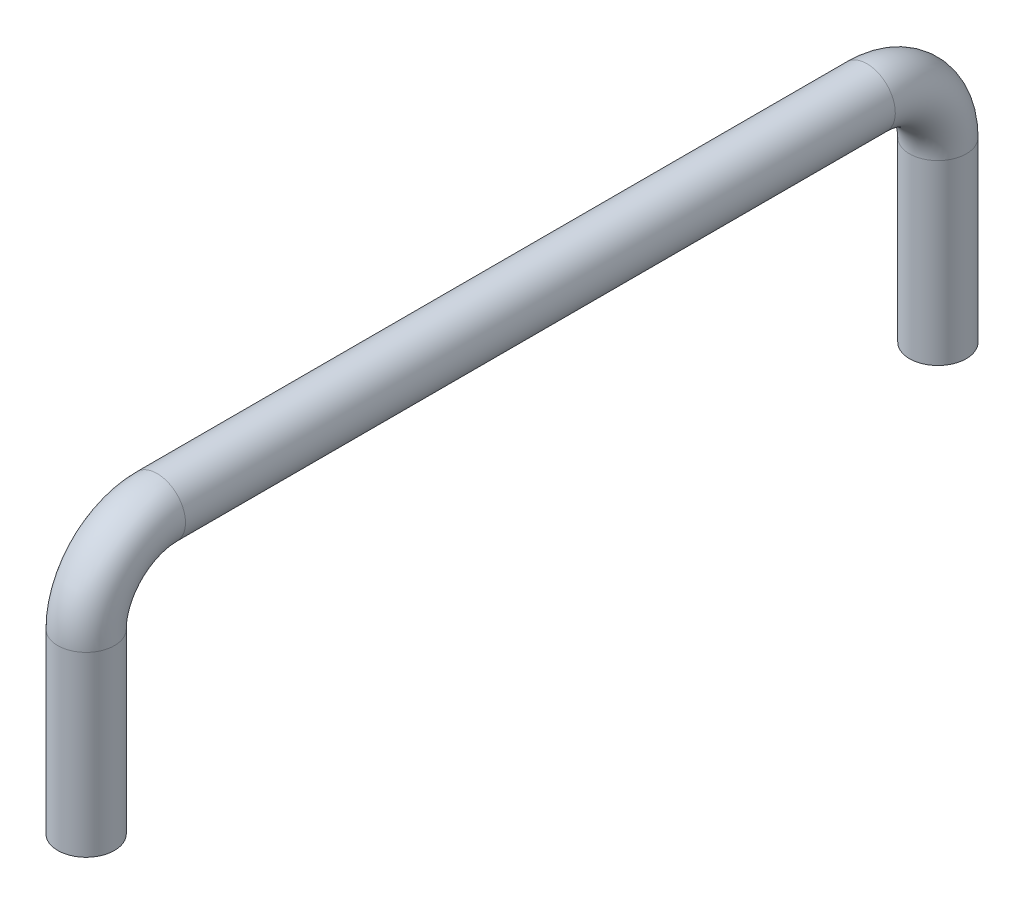
from build123d import *

# Parameters (mm, degrees)
SKETCH2_R = 5.08


with BuildPart() as part:
    # Sweep1: sweep along a path in Sketch1
    with BuildLine(Plane(origin=(0, 0, 0), x_dir=(0, 0, -1), z_dir=(1, 0, 0))) as sweep1_path:
        Line((-76.2, 57.15), (-76.2, 88.9))
        ThreePointArc((-76.2, 88.9), (-72.480256121, 97.880256121), (-63.5, 101.6))
        Line((-63.5, 101.6), (63.5, 101.6))
        ThreePointArc((63.5, 101.6), (72.480256121, 97.880256121), (76.2, 88.9))
        Line((76.2, 88.9), (76.2, 57.15))
    # Sketch2 → Sweep1 (sweep)
    with BuildSketch(Plane(origin=(0, 57.15, 76.2), x_dir=(-1, 0, 0), z_dir=(0, 1, 0))):
        Circle(SKETCH2_R)
    sweep(path=sweep1_path.line)


solid = part.part
